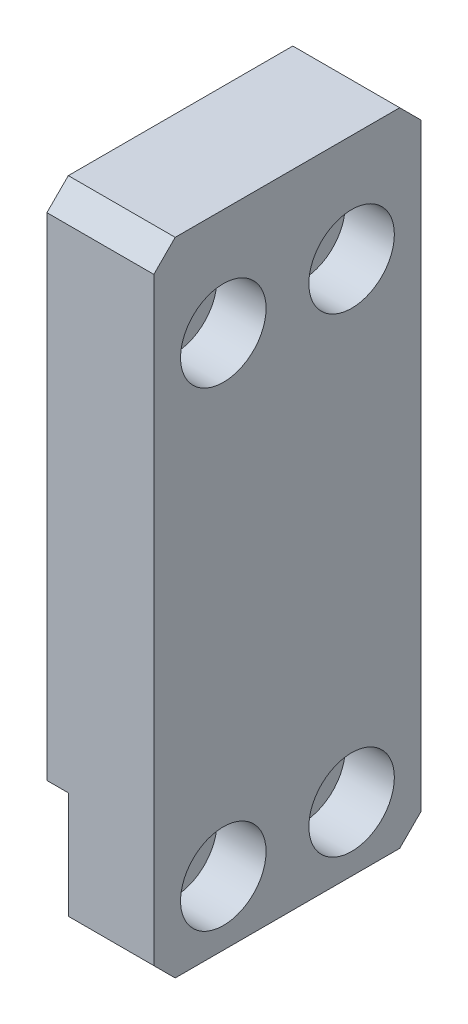
from build123d import *

# Parameters (mm, degrees)
SKETCH1_W                                            = 25
SKETCH1_H                                            = 60
BOSS_EXTRUDE1_DEPTH                                  = 10
SKETCH4_W                                            = 25
SKETCH4_H                                            = 12
CUT_EXTRUDE3_DEPTH                                   = 2
CBORE_FOR_M4_HEXAGON_SOCKET_HEAD_CAP_SCR_D           = 4.5
CBORE_FOR_M4_HEXAGON_SOCKET_HEAD_CAP_SCR_CBORE_D     = 8
CBORE_FOR_M4_HEXAGON_SOCKET_HEAD_CAP_SCR_CBORE_DEPTH = 4.6
CBORE_FOR_M4_HEXAGON_SOCKET_HEAD_CAP_2_D             = 4.5
CBORE_FOR_M4_HEXAGON_SOCKET_HEAD_CAP_2_CBORE_D       = 8
CBORE_FOR_M4_HEXAGON_SOCKET_HEAD_CAP_2_CBORE_DEPTH   = 4.6
CHAMFER1_SIZE                                        = 2


with BuildPart() as part:
    # Sketch1 → Boss-Extrude1 (new body)
    with BuildSketch(Plane(origin=(0, 0, 0), x_dir=(0, 0, -1), z_dir=(1, 0, 0))):
        Rectangle(SKETCH1_W, SKETCH1_H)
    extrude(amount=BOSS_EXTRUDE1_DEPTH)

    # Sketch4 → Cut-Extrude3 (cut)
    with BuildSketch(Plane.ZY):
        with Locations((0, -24)):
            Rectangle(SKETCH4_W, SKETCH4_H)
    extrude(amount=-CUT_EXTRUDE3_DEPTH, mode=Mode.SUBTRACT)

    # CBORE for M4 Hexagon socket head cap scr (through all)
    with Locations(Plane(origin=(10, 0, 0), x_dir=(0, 0, -1), z_dir=(1, 0, 0))):
        with Locations((-6, -24), (6, -24)):
            CounterBoreHole(CBORE_FOR_M4_HEXAGON_SOCKET_HEAD_CAP_SCR_D / 2, CBORE_FOR_M4_HEXAGON_SOCKET_HEAD_CAP_SCR_CBORE_D / 2, CBORE_FOR_M4_HEXAGON_SOCKET_HEAD_CAP_SCR_CBORE_DEPTH)

    # CBORE for M4 Hexagon socket head cap 2 (through all)
    with Locations(Plane(origin=(10, 0, 0), x_dir=(0, 0, -1), z_dir=(1, 0, 0))):
        with Locations((6, 20), (-6, 20)):
            CounterBoreHole(CBORE_FOR_M4_HEXAGON_SOCKET_HEAD_CAP_2_D / 2, CBORE_FOR_M4_HEXAGON_SOCKET_HEAD_CAP_2_CBORE_D / 2, CBORE_FOR_M4_HEXAGON_SOCKET_HEAD_CAP_2_CBORE_DEPTH)

    # Chamfer1
    chamfer1_edges = [part.edges().sort_by_distance(p)[0] for p in [
        (6, -30, -12.5),
        (6, -30, 12.5),
        (5, 30, 12.5),
        (5, 30, -12.5),
    ]]
    chamfer(chamfer1_edges, length=CHAMFER1_SIZE)


solid = part.part
